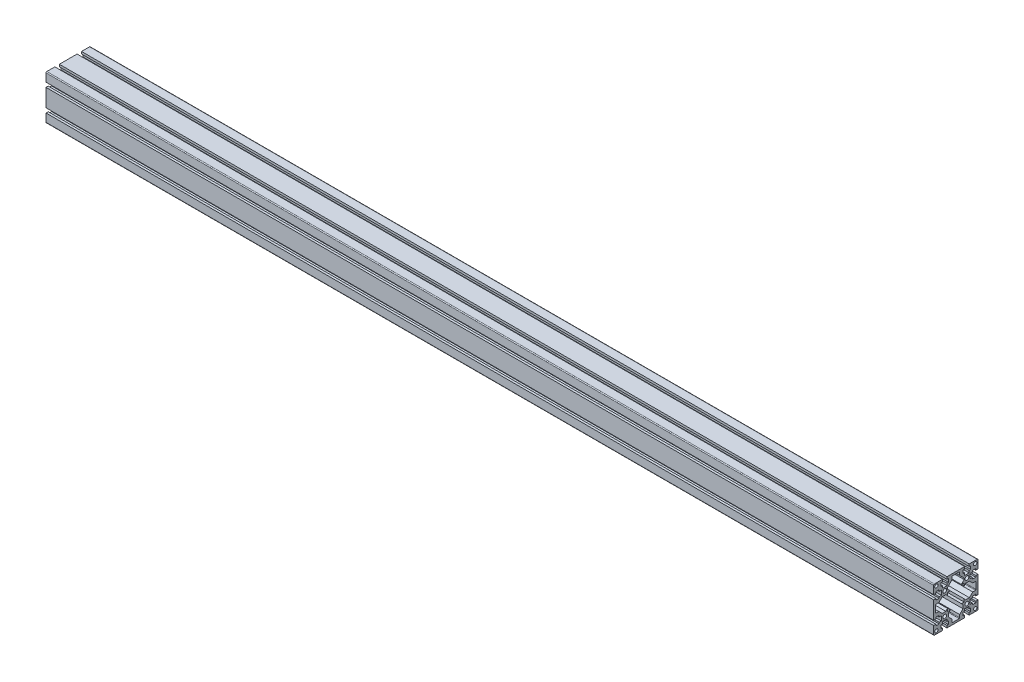
from build123d import *

# Parameters (mm, degrees)
SKETCH1_R                                = 3.4
SKETCH1_R_2                              = 3
ALUMINUM_PROFILE_80_X_80G_X_R1_5_1_DEPTH = 1600
SKETCH10_R                               = 3
CUT_EXTRUDE1_DEPTH                       = 1601.999687695


with BuildPart() as part:
    # Sketch1 → Aluminum profile 80 X 80G X R1.5(1) (new body)
    with BuildSketch(Plane.YZ.offset(-530.344827586)):
        with BuildLine():
            Line((-24.05, 40), (-24.05, 36))
            Line((-24.05, 36), (-26.75, 36))
            Line((-26.75, 36), (-26.75, 30))
            Line((-26.75, 30), (-24.05, 30))
            Line((-24.05, 30), (-24.05, 26))
            Line((-24.05, 26), (-15.95, 26))
            Line((-15.95, 26), (-15.95, 30))
            Line((-15.95, 30), (-13.25, 30))
            Line((-13.25, 30), (-13.25, 36))
            Line((-13.25, 36), (-15.95, 36))
            Line((-15.95, 36), (-15.95, 40))
            Line((-15.95, 40), (15.95, 40))
            Line((15.95, 40), (15.95, 36))
            Line((15.95, 36), (13.25, 36))
            Line((13.25, 36), (13.25, 30))
            Line((13.25, 30), (15.95, 30))
            Line((15.95, 30), (15.95, 26))
            Line((15.95, 26), (24.05, 26))
            Line((24.05, 26), (24.05, 30))
            Line((24.05, 30), (26.75, 30))
            Line((26.75, 30), (26.75, 36))
            Line((26.75, 36), (24.05, 36))
            Line((24.05, 36), (24.05, 40))
            Line((24.05, 40), (38.5, 40))
            ThreePointArc((38.5, 40), (39.560660172, 39.560660172), (40, 38.5))
            Line((40, 38.5), (40, 24.05))
            Line((40, 24.05), (36, 24.05))
            Line((36, 24.05), (36, 26.75))
            Line((36, 26.75), (30, 26.75))
            Line((30, 26.75), (30, 24.05))
            Line((30, 24.05), (26, 24.05))
            Line((26, 24.05), (26, 15.95))
            Line((26, 15.95), (30, 15.95))
            Line((30, 15.95), (30, 13.25))
            Line((30, 13.25), (36, 13.25))
            Line((36, 13.25), (36, 15.95))
            Line((36, 15.95), (40, 15.95))
            Line((40, 15.95), (40, -15.95))
            Line((40, -15.95), (36, -15.95))
            Line((36, -15.95), (36, -13.25))
            Line((36, -13.25), (30, -13.25))
            Line((30, -13.25), (30, -15.95))
            Line((30, -15.95), (26, -15.95))
            Line((26, -15.95), (26, -24.05))
            Line((26, -24.05), (30, -24.05))
            Line((30, -24.05), (30, -26.75))
            Line((30, -26.75), (36, -26.75))
            Line((36, -26.75), (36, -24.05))
            Line((36, -24.05), (40, -24.05))
            Line((40, -24.05), (40, -38.5))
            ThreePointArc((40, -38.5), (39.560660172, -39.560660172), (38.5, -40))
            Line((38.5, -40), (24.05, -40))
            Line((24.05, -40), (24.05, -36))
            Line((24.05, -36), (26.75, -36))
            Line((26.75, -36), (26.75, -30))
            Line((26.75, -30), (24.05, -30))
            Line((24.05, -30), (24.05, -26))
            Line((24.05, -26), (15.95, -26))
            Line((15.95, -26), (15.95, -30))
            Line((15.95, -30), (13.25, -30))
            Line((13.25, -30), (13.25, -36))
            Line((13.25, -36), (15.95, -36))
            Line((15.95, -36), (15.95, -40))
            Line((15.95, -40), (-15.95, -40))
            Line((-15.95, -40), (-15.95, -36))
            Line((-15.95, -36), (-13.25, -36))
            Line((-13.25, -36), (-13.25, -30))
            Line((-13.25, -30), (-15.95, -30))
            Line((-15.95, -30), (-15.95, -26))
            Line((-15.95, -26), (-24.05, -26))
            Line((-24.05, -26), (-24.05, -30))
            Line((-24.05, -30), (-26.75, -30))
            Line((-26.75, -30), (-26.75, -36))
            Line((-26.75, -36), (-24.05, -36))
            Line((-24.05, -36), (-24.05, -40))
            Line((-24.05, -40), (-38.5, -40))
            ThreePointArc((-38.5, -40), (-39.560660172, -39.560660172), (-40, -38.5))
            Line((-40, -38.5), (-40, -24.05))
            Line((-40, -24.05), (-36, -24.05))
            Line((-36, -24.05), (-36, -26.75))
            Line((-36, -26.75), (-30, -26.75))
            Line((-30, -26.75), (-30, -24.05))
            Line((-30, -24.05), (-26, -24.05))
            Line((-26, -24.05), (-26, -15.95))
            Line((-26, -15.95), (-30, -15.95))
            Line((-30, -15.95), (-30, -13.25))
            Line((-30, -13.25), (-36, -13.25))
            Line((-36, -13.25), (-36, -15.95))
            Line((-36, -15.95), (-40, -15.95))
            Line((-40, -15.95), (-40, 15.95))
            Line((-40, 15.95), (-36, 15.95))
            Line((-36, 15.95), (-36, 13.25))
            Line((-36, 13.25), (-30, 13.25))
            Line((-30, 13.25), (-30, 15.95))
            Line((-30, 15.95), (-26, 15.95))
            Line((-26, 15.95), (-26, 24.05))
            Line((-26, 24.05), (-30, 24.05))
            Line((-30, 24.05), (-30, 26.75))
            Line((-30, 26.75), (-36, 26.75))
            Line((-36, 26.75), (-36, 24.05))
            Line((-36, 24.05), (-40, 24.05))
            Line((-40, 24.05), (-40, 38.5))
            ThreePointArc((-40, 38.5), (-39.560660172, 39.560660172), (-38.5, 40))
            Line((-38.5, 40), (-24.05, 40))
        make_face()
        with Locations((-20, 20)):
            Circle(SKETCH1_R, mode=Mode.SUBTRACT)
        with Locations((20, 20)):
            Circle(SKETCH1_R, mode=Mode.SUBTRACT)
        with Locations((20, -20)):
            Circle(SKETCH1_R, mode=Mode.SUBTRACT)
        with Locations((-20, -20)):
            Circle(SKETCH1_R, mode=Mode.SUBTRACT)
        with Locations((-35, 35)):
            Circle(SKETCH1_R_2, mode=Mode.SUBTRACT)
        with Locations((35, 35)):
            Circle(SKETCH1_R_2, mode=Mode.SUBTRACT)
        with Locations((35, -35)):
            Circle(SKETCH1_R_2, mode=Mode.SUBTRACT)
        with BuildLine():
            Line((-13, 18), (-10, 15))
            Line((-10, 15), (-15, 15))
            Line((-15, 15), (-15, 10))
            Line((-15, 10), (-18, 13))
            Line((-18, 13), (-24.5, 13))
            Line((-24.5, 13), (-30.5, 7))
            Line((-30.5, 7), (-35.5, 7))
            ThreePointArc((-35.5, 7), (-36.207106781, 6.707106781), (-36.5, 6))
            Line((-36.5, 6), (-36.5, -6))
            ThreePointArc((-36.5, -6), (-36.207106781, -6.707106781), (-35.5, -7))
            Line((-35.5, -7), (-30.5, -7))
            Line((-30.5, -7), (-24.5, -13))
            Line((-24.5, -13), (-18, -13))
            Line((-18, -13), (-15, -10))
            Line((-15, -10), (-15, -15))
            Line((-15, -15), (-10, -15))
            Line((-10, -15), (-13, -18))
            Line((-13, -18), (-13, -24.5))
            Line((-13, -24.5), (-7, -30.5))
            Line((-7, -30.5), (-7, -35.5))
            ThreePointArc((-7, -35.5), (-6.707106781, -36.207106781), (-6, -36.5))
            Line((-6, -36.5), (6, -36.5))
            ThreePointArc((6, -36.5), (6.707106781, -36.207106781), (7, -35.5))
            Line((7, -35.5), (7, -30.5))
            Line((7, -30.5), (13, -24.5))
            Line((13, -24.5), (13, -18))
            Line((13, -18), (10, -15))
            Line((10, -15), (15, -15))
            Line((15, -15), (15, -10))
            Line((15, -10), (20, -15))
            Line((20, -15), (22.5, -15))
            Line((22.5, -15), (30.5, -7))
            Line((30.5, -7), (35.5, -7))
            ThreePointArc((35.5, -7), (36.207106781, -6.707106781), (36.5, -6))
            Line((36.5, -6), (36.5, 6))
            ThreePointArc((36.5, 6), (36.207106781, 6.707106781), (35.5, 7))
            Line((35.5, 7), (30.5, 7))
            Line((30.5, 7), (22.5, 15))
            Line((22.5, 15), (20, 15))
            Line((20, 15), (15, 10))
            Line((15, 10), (15, 15))
            Line((15, 15), (10, 15))
            Line((10, 15), (13, 18))
            Line((13, 18), (13, 24.5))
            Line((13, 24.5), (7, 30.5))
            Line((7, 30.5), (7, 35.5))
            ThreePointArc((7, 35.5), (6.707106781, 36.207106781), (6, 36.5))
            Line((6, 36.5), (-6, 36.5))
            ThreePointArc((-6, 36.5), (-6.707106781, 36.207106781), (-7, 35.5))
            Line((-7, 35.5), (-7, 30.5))
            Line((-7, 30.5), (-13, 24.5))
            Line((-13, 24.5), (-13, 18))
        make_face(mode=Mode.SUBTRACT)
    extrude(amount=ALUMINUM_PROFILE_80_X_80G_X_R1_5_1_DEPTH)

    # Sketch10 → Cut-Extrude1 (cut, through all)
    with BuildSketch(Plane(origin=(1069.655172414, 0, 0), x_dir=(0, 0, -1), z_dir=(1, 0, 0))):
        with Locations((35, -35)):
            Circle(SKETCH10_R)
    extrude(amount=-CUT_EXTRUDE1_DEPTH, mode=Mode.SUBTRACT)


solid = part.part
